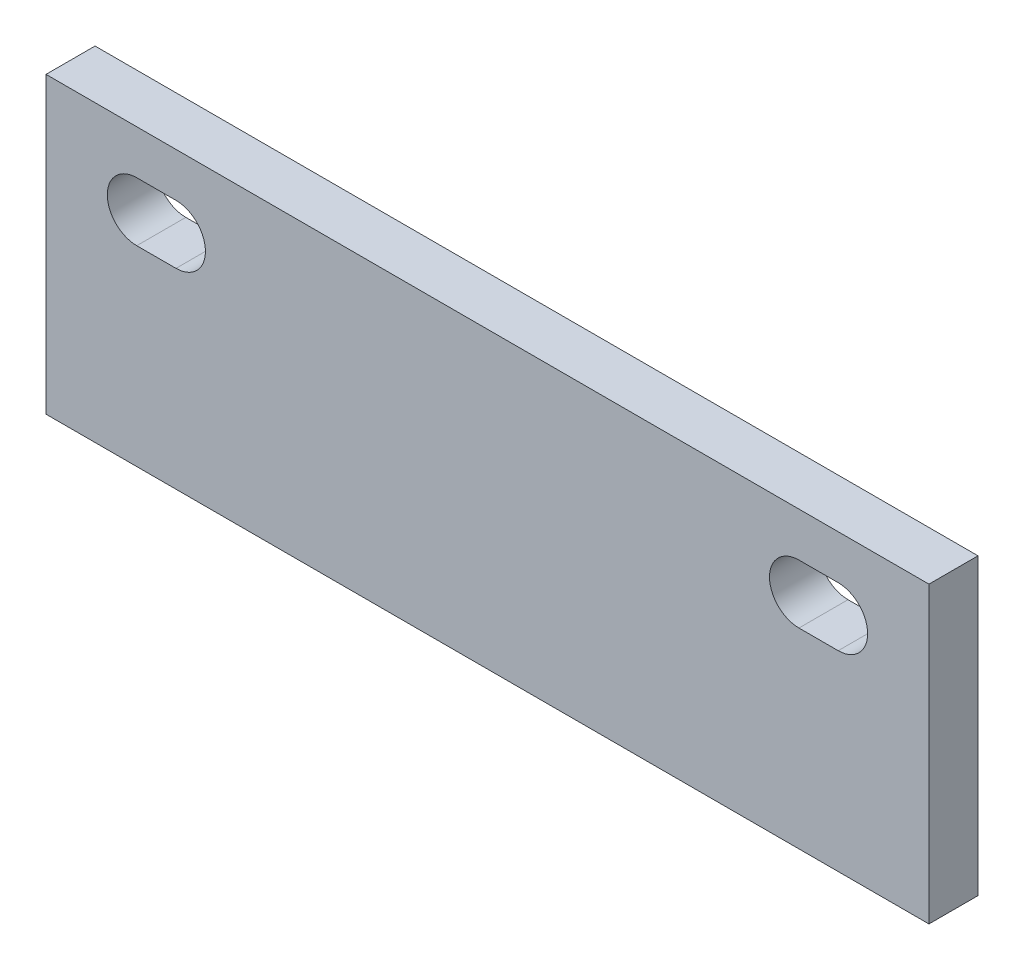
SolidWorks part; units mm, degrees
ref_plane "前视基准面" through (0, 0, 0) normal (0, 0, 1) x (1, 0, 0)
ref_plane "上视基准面" through (0, 0, 0) normal (0, 1, 0) x (1, 0, 0)
ref_plane "右视基准面" through (0, 0, 0) normal (1, 0, 0) x (0, 0, -1)
sketch "草图1" plane through (0, 0, 0) normal (0, 0, 1) x (1, 0, 0)
  line L0 (-90, 15) -> (90, 15) construction
  line L1 (-90, 30) -> (90, 30)
  line L2 (-90, 30) -> (-90, -30)
  line L3 (-90, -30) -> (90, -30)
  line L4 (90, 30) -> (90, -30)
  line L5 (-90, 30) -> (90, -30) construction
  line L6 (-90, -30) -> (90, 30) construction
  line L8 (-71.5, 21) -> (-63.5, 21)
  line L9 (-71.5, 21) -> (-71.5, 9) construction
  line L10 (-71.5, 9) -> (-63.5, 9)
  line L11 (-63.5, 21) -> (-63.5, 9) construction
  line L12 (-71.5, 21) -> (-63.5, 9) construction
  line L13 (-71.5, 9) -> (-63.5, 21) construction
  line L14 (63.5, 21) -> (71.5, 21)
  line L15 (63.5, 21) -> (63.5, 9) construction
  line L16 (63.5, 9) -> (71.5, 9)
  line L17 (71.5, 21) -> (71.5, 9) construction
  line L18 (63.5, 21) -> (71.5, 9) construction
  line L19 (63.5, 9) -> (71.5, 21) construction
  arc A0 (-71.5, 9) -> (-71.5, 21) centre (-71.5, 15) cw
  arc A1 (-63.5, 21) -> (-63.5, 9) centre (-63.5, 15) cw
  arc A2 (71.5, 21) -> (71.5, 9) centre (71.5, 15) cw
  arc A3 (63.5, 9) -> (63.5, 21) centre (63.5, 15) cw
  point P0 (0, 0)
  point P8 (-67.5, 15)
  point P16 (67.5, 15)
  dimension "D9" = 6
  dimension "D1" = 180
  dimension "D2" = 60
  dimension "D3" = 15
  dimension "D4" = 8
  dimension "D5" = 12
  dimension "D6" = 67.5
  dimension "D7" = 8
  dimension "D8" = 67.5
extrude "凸台-拉伸1" add sketch "草图1" along normal blind 10
